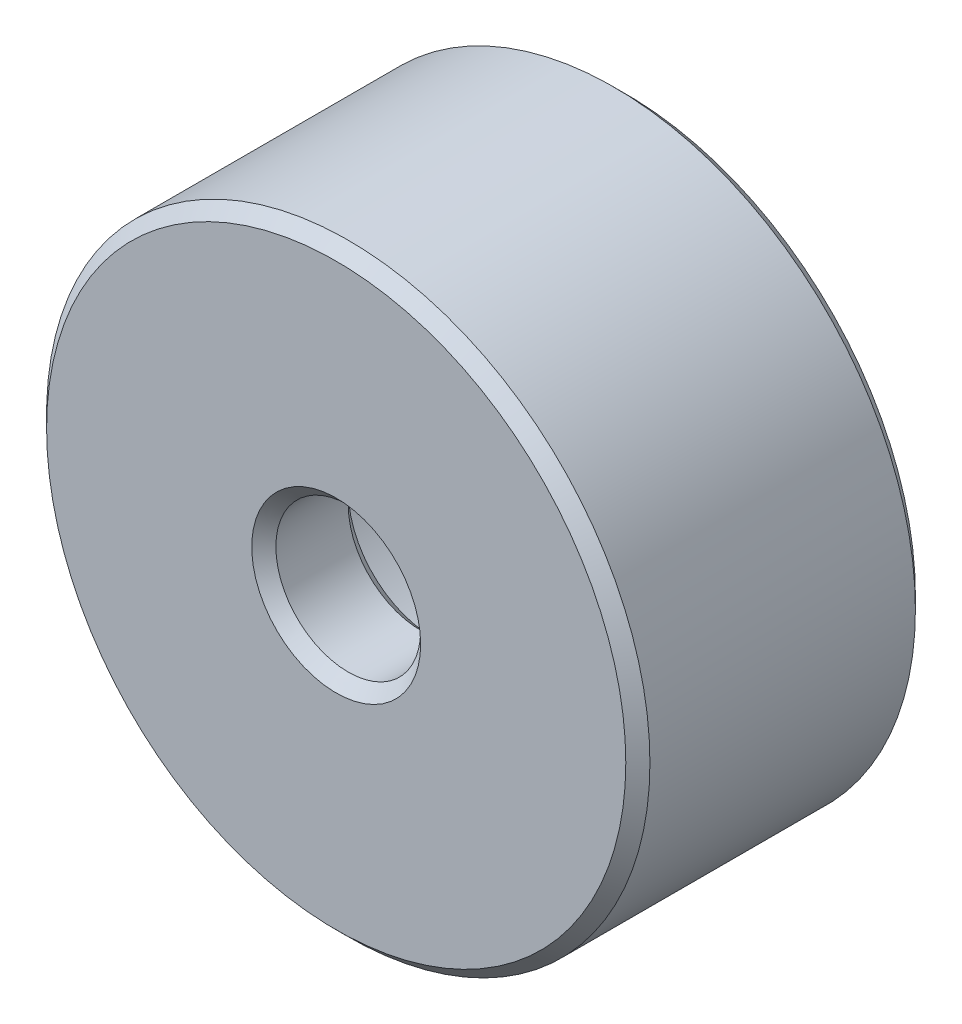
from build123d import *

# Parameters (mm, degrees)
SKETCH1_R           = 12.5
SKETCH1_R_2         = 3
BOSS_EXTRUDE1_DEPTH = 6
SKETCH2_R           = 8
CUT_EXTRUDE1_DEPTH  = 8
CHAMFER1_SIZE       = 0.5


with BuildPart() as part:
    # Sketch1 → Boss-Extrude1 (new, symmetric)
    with BuildSketch(Plane.XY):
        Circle(SKETCH1_R)
        Circle(SKETCH1_R_2, mode=Mode.SUBTRACT)
    extrude(amount=BOSS_EXTRUDE1_DEPTH, both=True)

    # Sketch2 → Cut-Extrude1 (cut)
    with BuildSketch(Plane(origin=(0, 0, -6), x_dir=(-1, 0, 0), z_dir=(0, 0, -1))):
        Circle(SKETCH2_R)
    extrude(amount=-CUT_EXTRUDE1_DEPTH, mode=Mode.SUBTRACT)

    # Chamfer1
    chamfer1_edges = [part.edges().sort_by_distance(p)[0] for p in [
        (-3, 0, 2),
        (8, 0, -6),
        (-12.5, 0, -6),
        (-12.5, 0, 6),
        (-3, 0, 6),
    ]]
    chamfer(chamfer1_edges, length=CHAMFER1_SIZE)


solid = part.part
